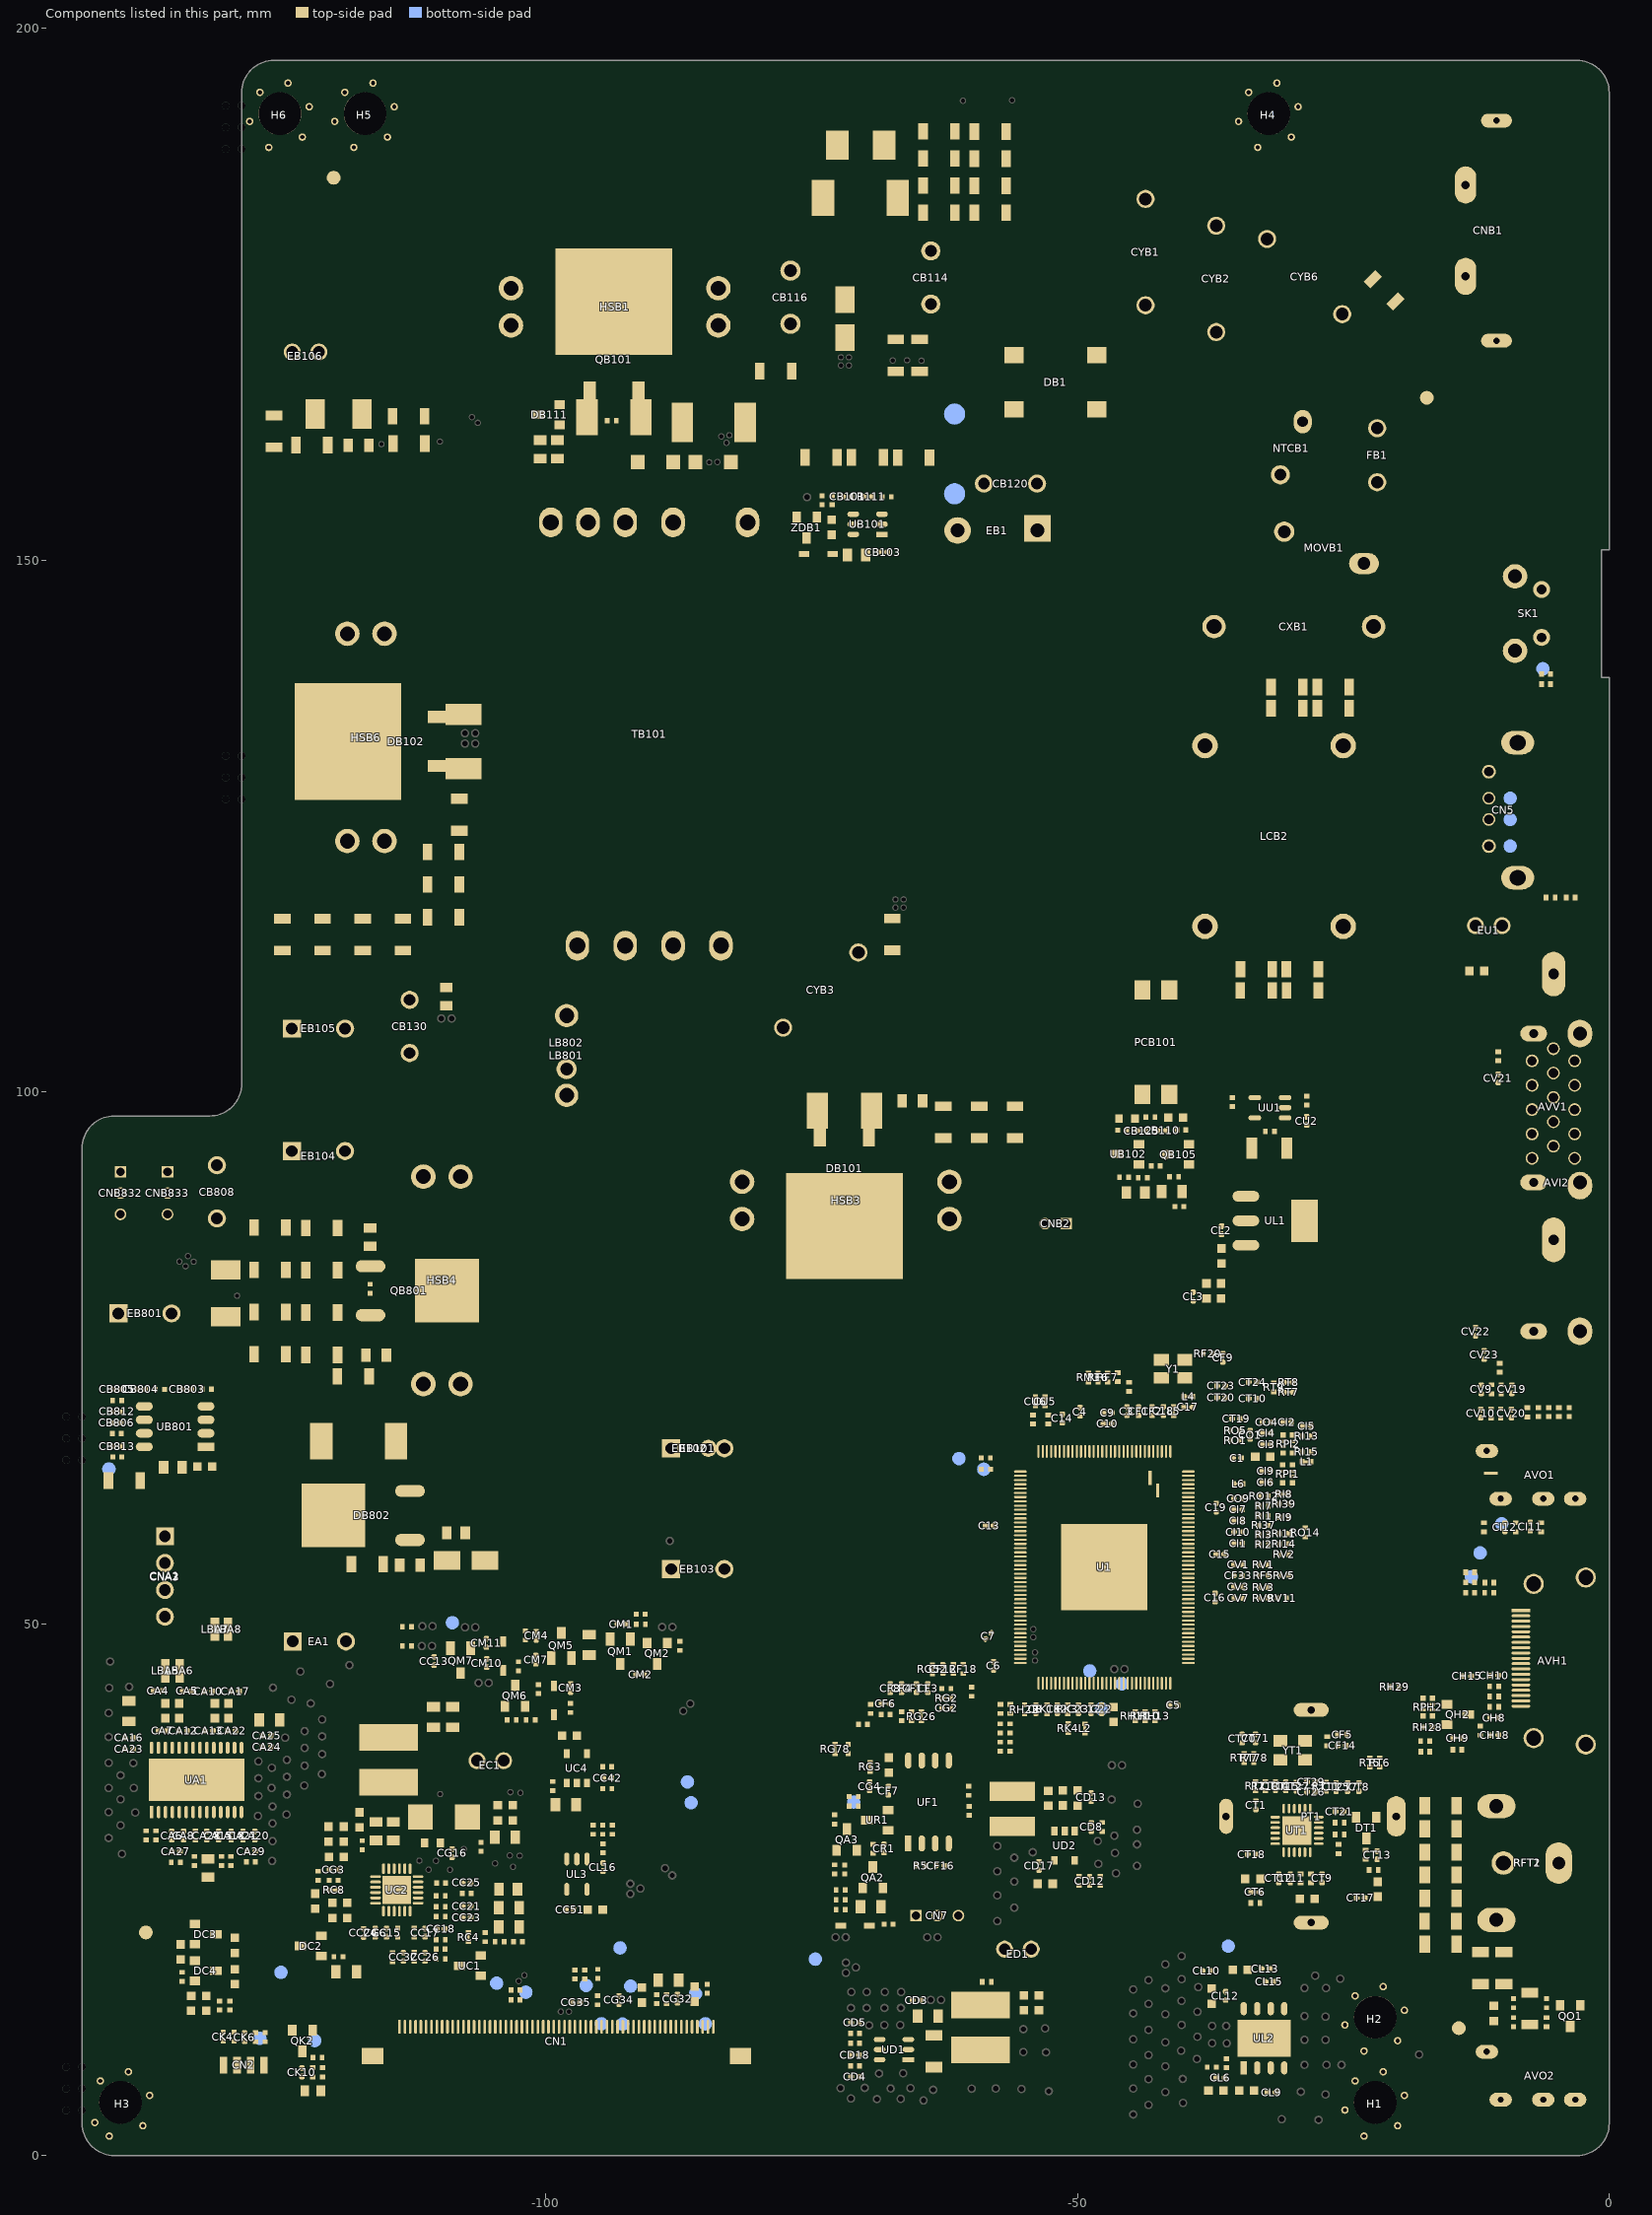
[diagram p0: the components of this part, seen from the top]
# Altium PCB MISC86383-9.PcbDoc (part 17 of 18)
Units mm, origin at the board's own origin, x right, y up, seen from the top; angles counter-clockwise.
Board outline 143.6 x 197 mm, 2 copper layers (TopLayer, BottomLayer), stack 1.571 mm thick; 743 components, 401 nets, 2996 pads, 1077 vias.
Unrouted connection lines stored in the file: 4.

## Other copper (continued)
BottomLayer:
  region net GND: -8.28,94.107 -8.28,94.539 -8.992,94.539 -8.992,94.107
  rectangle: 100.218,30.59 103.525,32.59
  rectangle net GND: -35.887,33.905 -35.444,34.127
  rectangle net GND: -30.734,18.072 -24.638,21.336
  rectangle net GND: -22.86,24.981 -17.036,34.29
  rectangle net GND: -33.02,18.923 -27.305,21.971
  rectangle net GND: -24.468,26.543 -20.955,33.267
  rectangle net GND: -31.191,20.206 -24.701,24.409
  rectangle net D_QB801: -100.546,96.622 -95.733,103.594
  rectangle net 12V: -83.756,84.9 -58.941,94.209
  rectangle net D_QB101: -79.172,175.882 -74.295,179.934
  rectangle net D_QB101: -88.113,169.799 -82.067,178.333
  rectangle net D_QB101: -105.118,169.659 -100.381,177.66
  rectangle net VBRIDGE: -54.839,158.064 -54.458,158.331
  rectangle net VBL: -123.368,116.853 -111.658,146.012
  rectangle net GND: -94.158,107.886 -88.849,110.299
  rectangle net GND: -91.364,70.193 -87.655,74.155
  rectangle net D_QB801: -113.474,90.094 -105.054,94.234
  rectangle net D_QB801: -113.017,70.904 -105.131,75.095
  region net 12V: -87.541,43.383 -87.541,41.618 -87.274,41.351 -86.906,41.351 -85.915,42.342 -85.915,42.913 -86.423,43.421 -86.893,43.421
  region net 12V: -89.357,48.87 -89.357,49.924 -89.179,50.102 -87.947,50.102 -87.693,49.847 -87.693,49.505 -88.455,48.743 -88.951,48.743
  region net AVDD: -102.984,16.535 -102.248,17.272 -101.879,17.272 -101.676,17.069 -101.676,16.535 -99.263,14.122 -97.815,14.122 -97.511,13.818 -97.511,13.03 -97.561,12.979 -99.695,12.979 -102.984,16.269
  region net 12V: -64.567,20.726 -64.338,20.955 -62.992,20.955 -62.763,20.726 -62.763,15.164 -62.408,14.808 -62.408,14.427 -62.636,14.199 -64.033,14.199 -64.237,14.402 -64.237,19.99 -64.567,20.32
  region net GND: -37.625,30.444 -37.625,33.559 -36.93,34.254 -36.014,34.254 -35.76,34 -35.478,34 -34.676,33.198 -34.744,33.13 -34.744,29.428 -36.339,29.428 -36.522,29.245 -36.705,29.428 -37.576,29.428
  region net 1.15V_STB: -46.899,45.216 -46.899,45.965 -46.676,46.189 -45.44,46.189 -45.187,45.936 -45.187,45.443 -46.112,44.518
  region net 1.15V_STB: -47.258,36.936 -46.951,37.243 -45.701,37.243 -45.396,36.938 -45.396,36.481 -45.657,36.22 -47.051,36.22 -47.258,36.427
  region net 1.15V_STB: -46.951,37.243 -46.069,38.125 -45.822,38.125 -45.822,37.008 -46.132,36.697 -46.768,36.697
  region net GND: -83.604,58.356 -71.247,58.356 -70.523,57.633 -76.468,51.688 -76.468,51.257 -79.565,51.257 -82.245,53.937 -82.245,54.191
  region net GND: -29.947,40.665 -29.947,42.202 -29.045,43.104 -26.54,43.104 -26.123,42.687 -26.123,41.527 -27.353,40.297 -29.54,40.297 -29.604,40.361
  pour cut-out: -25.349,41.859 -25.044,41.859 -24.956,41.948 -24.956,68.199 -25.021,68.264 -25.379,68.264 -25.379,67.814 -25.413,67.78 -25.349,67.716
  region net VBL: -120.294,108.267 -121.323,108.267 -123.33,106.261 -124.166,106.261 -124.166,106.54 -124.684,107.059 -123.114,108.629 -123.114,108.826
  region net NetCB113_1: -113.805,162.649 -118.554,162.649 -118.885,162.319 -118.885,160.045 -118.478,159.639 -113.982,159.639 -113.576,160.045 -113.576,162.42
  region net 12V-OVP: -111.709,162.649 -112.23,162.128 -112.23,160.007 -111.874,159.652 -109.182,159.652 -108.483,160.35 -108.483,162.166 -108.966,162.649
  region net NetDB104_K: -123.581,170.003 -124.485,170.003 -125.895,168.592 -125.895,162.382 -125.209,161.696 -120.866,161.696 -120.205,162.357 -120.205,165.062 -123.317,168.173 -123.317,169.739
  region net SGND: -82.461,161.722 -82.461,161.029 -82.334,160.902 -83.858,159.378 -83.858,159.245 -84.747,159.245 -84.849,159.347 -84.633,159.563 -84.633,160.782 -83.693,161.722
  pour cut-out: -74.409,151.6 -74.409,151.654 -74.683,151.928 -74.72,151.892 -75.463,151.892 -75.463,152.262 -76.148,152.946 -76.657,152.946 -76.657,152.044 -75.334,150.721 -75.017,150.721
  region net VBRIDGE: -63.36,167.018 -59.258,162.916 -63.449,162.916 -63.779,163.246 -63.665,163.36 -63.665,166.408
  region net VBRIDGE: -52.514,179.578 -56.413,179.578 -57.328,178.664 -57.328,173.584 -58.839,172.072 -58.839,166.98 -57.48,165.621 -54.889,165.621 -54.889,173.291 -52.197,175.984 -52.197,179.26
  region net NetCB114_1: -63.246,174.777 -64.287,174.777 -66.408,172.656 -67.437,172.656 -67.843,172.25 -67.843,170.447 -67.767,170.37 -64.732,170.37 -62.954,172.148 -62.954,174.485
  region net VBRIDGE: -61.735,165.557 -61.722,165.57 -61.722,170.65 -62.687,170.65 -64.364,168.973 -64.364,167.107 -62.967,165.71
  region net VBRIDGE: -64.364,169.177 -67.831,169.177 -68.135,168.872 -68.135,161.201 -68.529,160.807 -68.351,160.63 -64.046,160.63 -62.497,162.179 -62.497,167.157 -63.792,168.453
  region net VBRIDGE: -52.946,196.012 -57.048,196.012 -57.544,195.516 -57.544,183.515 -56.483,182.455 -53.391,185.547 -53.391,189.624 -52.159,190.856 -52.159,195.224
  region net NetRB150_1: -59.22,196.063 -62.154,196.063 -62.509,195.707 -62.509,184.455 -61.887,183.832 -59.398,183.832 -58.699,184.531 -58.699,195.542
  region net NetCB114_2: -64.173,195.885 -68.44,195.885 -69.266,195.059 -69.266,187.833 -67.843,186.411 -67.843,182.385 -64.122,178.664 -63.144,178.664 -63.144,178.981 -61.912,180.213 -61.912,180.861 -63.602,182.55 -63.602,195.313
  region net L: -47.981,172.758 -48.73,172.009 -50.66,172.009 -50.66,171.539 -50.228,171.107 -50.952,170.383 -50.952,169.367 -44.539,162.954 -44.539,168.186 -43.059,169.666 -45.047,171.653 -45.047,172.923
  region net L: -43.548,174.777 -48.628,174.777 -50.952,172.453 -50.952,169.367 -50.267,168.681 -45.555,168.681 -44.793,167.919 -44.475,168.237 -43.472,168.237 -43.472,169.253 -42.647,170.078 -42.672,170.104 -42.672,173.901
  region net N-2: -29.616,120.18 -29.388,120.18 -28.939,120.629 -28.939,120.811 -28.668,121.082 -26.302,121.082 -23.838,118.618 -23.838,115.341 -24.46,114.719 -25.565,114.719 -25.565,114.783 -27.127,116.345 -28.939,116.345 -28.939,120.811
  region net N: -33.244,120.78 -34.668,120.78 -39.027,116.421 -39.027,115.303 -38.519,114.795 -37.122,114.795 -37.122,114.833 -35.642,116.314 -33.244,116.314
  region net N: -33.244,119.647 -31.541,120.229 -33.244,120.78
  region net N: -33.244,118.539 -31.541,119.121 -33.244,119.672
  region net N: -33.244,116.314 -31.541,116.896 -33.244,117.447
  region net N: -33.244,117.431 -31.541,118.013 -33.244,118.564
  region net N-2: -28.939,119.694 -30.641,119.111 -28.939,118.56
  region net N-2: -28.939,120.811 -30.641,120.229 -28.939,119.678
  region net N-2: -28.939,118.586 -30.641,118.003 -28.939,117.453
  region net N-2: -28.939,117.478 -30.641,116.896 -28.939,116.345
  region net L-2: -25.375,137.617 -25.768,137.223 -25.768,135.547 -27.004,134.311 -28.85,134.311 -28.85,129.845 -28.571,129.565 -26.175,129.565 -23.736,132.004 -23.736,133.172
  region net L: -39.497,131.813 -39.446,131.864 -39.446,133.375 -38.837,133.375 -38.837,133.782 -38.338,134.28 -33.155,134.28 -33.155,133.993 -33.122,133.96 -33.155,133.926 -33.155,129.814 -37.497,129.814
  region net L: -33.155,133.147 -31.453,133.729 -33.155,134.28
  region net L: -33.155,132.039 -31.453,132.621 -33.155,133.172
  region net L: -33.155,129.814 -31.453,130.396 -33.155,130.947
  region net L: -33.155,130.931 -31.453,131.513 -33.155,132.064
  region net L-2: -28.85,133.194 -30.553,132.611 -28.85,132.06
  region net L-2: -28.85,134.311 -30.553,133.729 -28.85,133.178
  region net L-2: -28.85,132.086 -30.553,131.504 -28.85,130.953
  region net L-2: -28.85,130.978 -30.553,130.396 -28.85,129.845
  region net L-1: -20.904,168.783 -21.311,168.783 -23.089,167.005 -23.089,162.166 -22.479,161.557 -21.057,161.557 -19.837,162.776 -19.837,169.342 -20.041,169.545
  region net L-2: -22.593,158.217 -23.749,157.061 -23.749,151.066 -24.498,150.317 -24.498,145.936 -23.47,144.907 -23.47,142.913 -22.53,141.973 -22.034,142.469 -21.082,142.469 -21.082,155.423 -20.587,155.918 -20.587,157.442 -21.361,158.217
  region net L-1: -12.84,178.714 -14.402,178.714 -15.837,177.279 -15.837,175.565 -15.227,174.955 -13.31,174.955 -12.192,176.073 -12.192,178.067
  pour cut-out: -117.221,108.61 -117.221,110.211 -115.646,111.785 -104.877,111.785 -103.657,113.005 -103.657,111.061 -104.483,111.061 -105.677,109.868 -114.351,109.868
  region net LED_FB: -126.238,85.23 -127.178,85.23 -129.896,82.512 -129.896,76.365 -128.168,74.638 -126.352,74.638 -125.933,75.057 -125.933,84.925
  region net GND: -121.971,89.878 -125.235,89.878 -126.975,88.138 -126.975,86.335 -127.114,86.195 -127.013,86.093 -126.073,86.093 -125.539,85.56 -125.539,73.127 -125.311,72.898 -125.298,72.911 -122.276,72.911 -121.552,73.635 -121.552,89.459
  pour cut-out: -144.043,64.008 -143.51,64.008 -141.795,62.293 -141.795,62.078 -143.459,62.078 -144.272,62.89
  region net LED+: -127.851,71.971 -127.571,71.691 -116.192,71.691 -112.382,67.882 -112.382,58.306 -113.144,57.544 -120.739,57.544 -127.317,64.122 -127.317,70.929 -127.8,71.412
  region: -120.65,88.875 -118.91,88.875 -118.059,88.024 -118.059,74.308 -118.504,73.863 -120.409,73.863 -121.044,74.498 -121.044,88.481
  region: -65.138,100.381 -52.883,100.381 -52.387,99.885 -52.387,97.472 -52.73,97.13 -64.999,97.13 -65.405,97.536 -65.405,100.114
  pour cut-out: -14.402,116.332 -14.402,109.779 -23.876,100.305 -28.321,100.305 -28.321,102.413
  pour cut-out: 1.851,19.007 -12.859,19.007 cw(c-12.859,21.547) -15.399,21.547 -15.399,33.402 cw(c-12.859,33.402) -12.859,35.942 1.554,35.942 cw(c1.554,35.497) 1.999,35.497 1.999,34.246 cw(c1.789,34.246) 1.789,34.036 -11.278,34.036 ccw(c-11.278,31.773) -13.54,31.773 -13.54,23.094 ccw(c-11.346,23.094) -11.346,20.9 1.664,20.9 cw(c1.664,20.734) 1.83,20.734 1.83,19.375 ccw(c1.907,19.375) 1.907,19.297
  pour cut-out: -10.732,129.614 -8.395,129.614 cw(c-8.395,128.497) -7.605,129.287 cw(c-8.15,128.742) -7.379,128.742 -7.379,122.921 cw(c-8.69,122.921) -7.763,121.994 cw(c-8.145,122.376) -8.145,121.836 -10.512,121.836 cw(c-10.515,123.262) -11.522,122.254 cw(c-10.896,122.881) -11.782,122.881 -11.782,128.137 cw(c-10.124,128.137) -11.296,129.309 -11.025,129.58
  text ".GBL" at 114.829,31.141 h1.52
  text "BottomLayer" at 104.099,31.103 h1.52

## Silkscreen, mask and mechanical layers (free items; w line width, h text height)
TopOverlay:
  drawing of 287 lines, arcs and shapes, not listed
  text "Solder Mask:" at 96.792,162.119 h1.52
  text "IPC SM-840" at 107.269,162.094 h1.52
  text "Silkscreen Color:" at 126.726,162.094 h1.52
  text "White" at 138.892,162.094 h1.52
  text "Units:" at 126.726,159.579 h1.52
  text "PTH Copper Thickness:" at 96.792,159.554 h1.52
  text "mm" at 131.755,159.541 h1.52
  text ">20um" at 113.899,159.528 h1.52
  text "4.2 --- 4.6" at 126.743,157.052 h1.52
  text "Dielectric Constant Er@1GHz To 1MHz:" at 96.783,157.04 h1.52
  text "Panel Size:" at 96.741,154.537 h1.52
  text "2L,2,136.85×197.00mm,FR4(TG130-CTI175),1OZ,Green,OSP,1.6mm" at 104.492,154.538 h1.52
  text "Silkscreen on PTH:" at 96.754,151.959 h1.52
  text "Primary Side Retained;" at 109.911,151.934 h1.52
  text "Secondary Side  Removed for Soldering" at 126.726,151.896 h1.52
  text "KEY" at -9.309,151.193 h1.52
  text "Special Requirements" at 96.728,149.656 h1.52
  text "工程问题2小时内没回复，请电联" at 144.65,149.471 h1.52
  text "1. Lead-free HASL (HAL_LF, Lead Free Hot Air Leveling)" at 111.737,147.025 h1.52
  text "2. Organic Solderability Preservative (OSP, Organic Solderability Preservatives)" at 111.737,144.891 h1.52
  text "3. Electroless Nickel Immersion Gold (ENIG, Electroless Nickel/Immersion Gold)" at 111.699,142.567 h1.52
  text "Plated Technics" at 98.633,141.685 h1.52
  text "4. ENIG + gold finger (ENIG_G/F, Electroless Nickel/Immersion Gold + Gold Finger)" at 111.737,140.522 h1.52
  text "5. Gold plating (Gold_plated, Gold-plated)" at 111.762,138.478 h1.52
  text "6. Gold plating + gold finger (Gold_Plated_G/F, Gold-plated + Gold Finger)" at 111.775,136.496 h1.52
  text "2" at -269.061,132.451 h4.06 r270
  text "Impedance Control" at 96.849,130.69 h1.52
  text "Target Impedance" at 117.088,130.693 h1.52
  text "Width & Clearance" at 136.032,130.687 h1.52
  text "Layer(s)" at 155.547,130.695 h1.52
  text "75 +/- 10% Ohm" at 117.411,127.995 h1.52
  text "G/12/14.5/12/G mil" at 134.709,127.978 h1.52
  text "layer 1" at 155.306,127.981 h1.52
  text "Single End Impedance" at 96.849,126.961 h1.52
  text "75 +/- 10% Ohm" at 117.411,125.506 h1.52
  text "G/7/6.9/7/G mil" at 134.709,125.489 h1.52
  text "layer 1" at 155.306,125.492 h1.52
  text "[ Zo ]" at 102.526,123.475 h1.52
  text "G/5/6.1/5/6.1/5/G mil" at 134.963,118.046 h1.52
  text "100 +/- 10% Ohm" at 117.081,118.021 h1.52
  text "layer 1" at 155.585,117.976 h1.52
  text "Differential Impedance" at 96.845,116.761 h1.52
  text "90 +/- 10% Ohm" at 117.704,115.646 h1.52
  text "layer 1" at 155.445,115.626 h1.52
  text "G/5/9.2/5/9.2/5/G mil" at 134.925,115.557 h1.52
  text "[ Zo ]" at 102.513,113.628 h1.52
  text "( G: Ground )" at 100.229,110.898 h1.52
  text "Common Mode Impedance" at 96.331,105.267 h1.52
  text "[ Zc ]" at 102.631,103.209 h1.52
  text "Refer to Gerber documents GTP&GBP for Stencil aperture design" at 119.574,96.499 h1.52
  text "Stencil (Stencil)" at 96.694,94.035 h1.52
  text "New" at 119.52,91.557 h1.52
  text "Test fixture (Testing jig)" at 96.646,89.066 h1.52
  text "New" at 119.551,89.041 h1.52
  text "Wave-soldering fixture (Wave-soldering jig)" at 96.702,86.57 h1.52
  text "New" at 119.573,86.574 h1.52
  text "Solder paste" at 119.511,83.985 h1.52
  text "Production process" at 96.664,83.947 h1.52
  text "[Process and notes]" at 101.241,81.792 h1.52
  text "Special requirements (Special Requirements)" at 96.689,78.918 h1.52
  text "SMD parts over 2mm high on wave-solder side" at 96.682,76.344 h1.52
  text "Packaging notes (Package Attention)" at 96.673,73.9 h1.52
  text "[Easily damaged components]" at 102.803,71.747 h1.52
  text "JX label" at -20.015,69.393 h3 r90
  text "New footprint matching (Footprint Matching)" at 96.673,68.82 h1.52
  text "[New component footprint]" at 102.448,66.692 h1.52
  text "1" at -4.209,63.952 h4.06 r90
  text "(Automated Testing Support)" at 104.759,63.784 h1.14
  text "Automatic test support" at 96.669,63.695 h1.52
  text "[Reserved suction cup and press pin positions]" at 100.746,61.548 h1.52
  text "Layer Stack Up Detail for" at 100.253,52.416 h2.54
  text ".Pcb_File_Name_No_Path" at 127.198,52.416 h2.54
  text "SPEAKER" at -128.118,50.495 h1.52 r90
  text "Layer" at 104.428,48.664 h1.27
  text "Gerber" at 113.869,48.664 h1.27
  text "Layer" at 121.772,48.664 h1.27
  text "Layer" at 137.933,48.664 h1.27
  text "Copper" at 157.971,48.664 h1.27
  text "Dielectric" at 165.89,48.664 h1.27
  text "Stack up" at 137.933,47.372 h1.27
  text "Height" at 165.89,47.372 h1.27
  text "Name" at 104.428,47.334 h1.27
  text "Document" at 113.869,47.334 h1.27
  text "Ordor" at 121.772,47.334 h1.27
  text "Thickness" at 157.971,47.334 h1.27
  text "TopOverlay" at 104.42,41.419 h1.52
  text ".GTO" at 114.823,41.354 h1.52
  text "0.4mil" at 165.822,39.194 h1.52
  text "1" at 123.124,36.574 h1.52
  text "1.4mil" at 158.303,36.573 h1.52
  text "2" at 123.125,31.163 h1.52
  text "1.4mil" at 158.259,31.138 h1.52
  text "0.4mil" at 165.89,28.733 h1.52
  text "UART" at -66.573,18.542 h1.52
  text "V1 2019.12.23" at -74.422,15.875 h2.54 r90
  text "TCON" at -79.629,9.779 h1.52
  text "IR" at -133.985,9.144 h1.52
  text "LED" at -119.888,5.715 h1.52
BottomOverlay:
  circle w0.127: c-32,192 r9.5
  circle w0.127: c-32,192 r17
  circle w0.127: c-32,192 r19
  circle w0.127: c-32,192 r9.5
  rectangle: 100.218,25.719 103.525,27.719
  lines w0.127: -137.114,49.662 -141.883,49.662 -141.883,58.932 -141.883,59.484 -136.886,59.484 ; -125,201.5 ccw(c-125,192) -125,182.5 -117,182.5 ccw(c-117,192) -117,201.5 ; -125,209 ccw(c-125,192) -125,175 -117,175 ccw(c-117,192) -117,209 ; -125,211 ccw(c-125,192) -125,173 -117,173 ccw(c-117,192) -117,211 ; -66.497,21.158 -66.497,17.526 -59.893,17.526 -59.893,21.158 ; 114.211,25.719 114.211,27.719 ; -50.461,16.744 -39.961,16.744 -39.961,27.244 -50.461,27.244 -50.461,16.744 ; -12.76,41.225 -2.26,41.225 -2.26,51.725 -12.76,51.725 -12.76,41.225 ; 100.218,25.719 118.812,25.719 118.812,27.719 100.218,27.719 100.218,25.719
  text "USB IN" at -2.07,123.368 h1.52 r270
  text "VGA IN" at -1.564,96.202 h1.52 r270
  text "AV2 IN" at -1.981,84.303 h1.52 r270
  text "AV OUT(mini)" at -1.168,66.929 h1.52
  text "AV1 IN(mini)" at -1.168,65.468 h1.52
  text "ROUT+" at -137.808,57.861 h1.27
  text "ROUT-" at -137.782,55.448 h1.27
  text "LOUT-" at -137.77,52.946 h1.27
  text "LOUT+" at -137.782,50.736 h1.27
  text "HDMI (ARC&UART) IN" at -1.508,39.447 h1.52 r270
  text ".GBO" at 114.839,26.304 h1.52
  text "BottomOverlay" at 104.129,26.279 h1.52
  text "RF IN" at -2.502,25.59 h1.52 r270
  text "GND" at -65.659,18.288 h1.27 r270
  text "RX" at -63.373,18.288 h1.27 r270
  text "TX" at -61.595,18.288 h1.27 r270
  text "V1 2019.12.23" at -82.423,15.113 h2.54 r270
  text "XCM101B1-PT" at -79.883,15.113 h2.54 r270
  text "EXT-IR" at -3.848,9.169 h1.52
TopPaste:
  rectangle: 100.218,43.332 103.525,45.332
  lines w0.127: 114.211,43.332 114.211,45.332 ; 100.218,43.332 100.218,45.332 118.812,45.332 118.812,43.332 100.218,43.332
  text "TopPaste" at 104.42,43.871 h1.52
  text ".GTP" at 114.823,43.817 h1.52
BottomPaste:
  rectangle: 100.218,23.328 103.525,25.328
  lines w0.127: 114.211,23.328 114.211,25.328 ; 100.218,23.328 100.218,25.328 118.812,25.328 118.812,23.328 100.218,23.328
  text "BottomPaste" at 104.099,23.912 h1.52
  text ".GBP" at 114.846,23.781 h1.52
TopSolder:
  rectangle: 100.218,38.507 103.525,40.507
  lines w0.127: 114.211,38.507 114.211,40.507 ; 100.218,38.507 100.218,40.507 118.812,40.507 118.812,38.507 100.218,38.507
  text "TopSolder" at 104.433,39.018 h1.52
  text ".GTS" at 114.823,38.976 h1.52
BottomSolder:
  rectangle: 100.218,28.098 103.525,30.098
  region: -29.047,116.134 -29.047,120.934 -33.147,120.934 -33.147,116.134
  region: -28.958,129.634 -28.958,134.434 -33.058,134.434 -33.058,129.634
  region: -11.642,93.166 -8.642,93.166 -8.642,103.542 -11.642,103.542
  lines w0.127: 114.211,28.098 114.211,30.098 ; 100.218,28.098 100.218,30.098 118.812,30.098 118.812,28.098 100.218,28.098
  lines w0.7: -10.206,43.779 -4.827,49.158 ; -10.204,45.902 -6.931,49.175 ; -10.204,48.024 -9.053,49.175 ; -8.086,43.777 -4.819,47.045 ; -5.965,43.777 -4.819,44.923
  lines w1: -49.803,17.401 -40.635,26.57 ; -49.803,20.23 -43.463,26.57 ; -49.803,23.058 -46.292,26.57 ; -49.803,25.887 -49.12,26.57 ; -46.988,17.388 -40.655,23.722 ; -44.164,17.384 -40.655,20.893 ; -41.347,17.373 -40.655,18.065
  text "BottomSolder" at 104.099,28.646 h1.52
  text ".GBS" at 114.822,28.624 h1.52
过炉治具:
  lines w0.5: -0.368,153.403 -0.368,198.691 3.01,198.691
  lines w2.1: -103.911,143.51 -104.483,143.51 -106.134,141.859 -106.134,139.014 -105.689,138.57 -101.765,138.57 ; -101.079,123.901 -106.134,123.901 -106.134,119.609 -99.606,119.609
  lines w3: -46.444,127.889 -46.444,138.379
  lines w3.2: -25.679,158.788 -25.679,164.846 -22.06,168.465
  lines w4: -7.823,167.843 -12.662,167.843 -14.186,169.367 -14.186,171.755 -12.484,173.457 -5.918,173.457
  lines w5: -22.466,181.496 -22.466,182.245
  lines w8: -126.568,154.203 -112.357,154.203 -101.092,142.938 -80.194,142.938 -75.641,138.386 -75.641,111.112 -69.266,104.737 -46.469,104.737 ; -46.52,203.403 -46.52,188.785 -48.603,186.703 -48.603,181.813 -45.758,178.968 -41.427,178.968 -38.887,176.428 -35.128,176.428 -34.011,175.311 -30.061,175.311 -24.257,181.115 -24.257,182.207 -19.139,187.325 -19.139,197.294 -16.472,199.961 -16.472,205.13 ; -43.967,104.572 -25.578,104.572 -18.86,111.29 -18.86,135.026 -15.811,138.074 -15.811,154.292 -5.905,164.198 7.175,164.198
3D和装配:
  lines w0.127: -273.7,193.5 -273.7,197 -270.7,197 ; -148.1,0 -145.1,0 -145.1,3 ; -143.6,3.175 -143.6,0 -140.6,0 ; -3.549,197 0,197 0,193.412 ; 0,3.016 0,0 ; 0,3.213 0,0 ; -3,0 0,0 ; -3,0 0,0 ; -3,0 0,0 ; 0,0 0,3.5 ; 0,0 0,3.5 ; 0,0 -2.997,0 0,0 ; 0,0 0,3.5 ; -51.961,15.244 -51.961,28.744 -38.461,28.744 -38.461,15.244 -51.961,15.244 ; -14.26,39.725 -0.76,39.725 -0.76,53.225 -14.26,53.225 -14.26,39.725
  lines w1.8: 3.912,17.628 -15.138,17.628 -15.863,18.352 -15.863,34.48 -15.342,35.001 -12.04,35.001 7.772,35.001
  text "2L,2,136.85×197.00mm,FR4(TG130-CTI175),1OZ,Green,OSP,1.6mm,5,40,83.2%,5.55,0.4mm" at 104.492,154.538 h1.52
端子视图:
  lines w1.8: 5.639,19.93 -12.564,19.93 -14.478,21.844 -14.478,33.071 -12.548,35.001 9.042,35.001